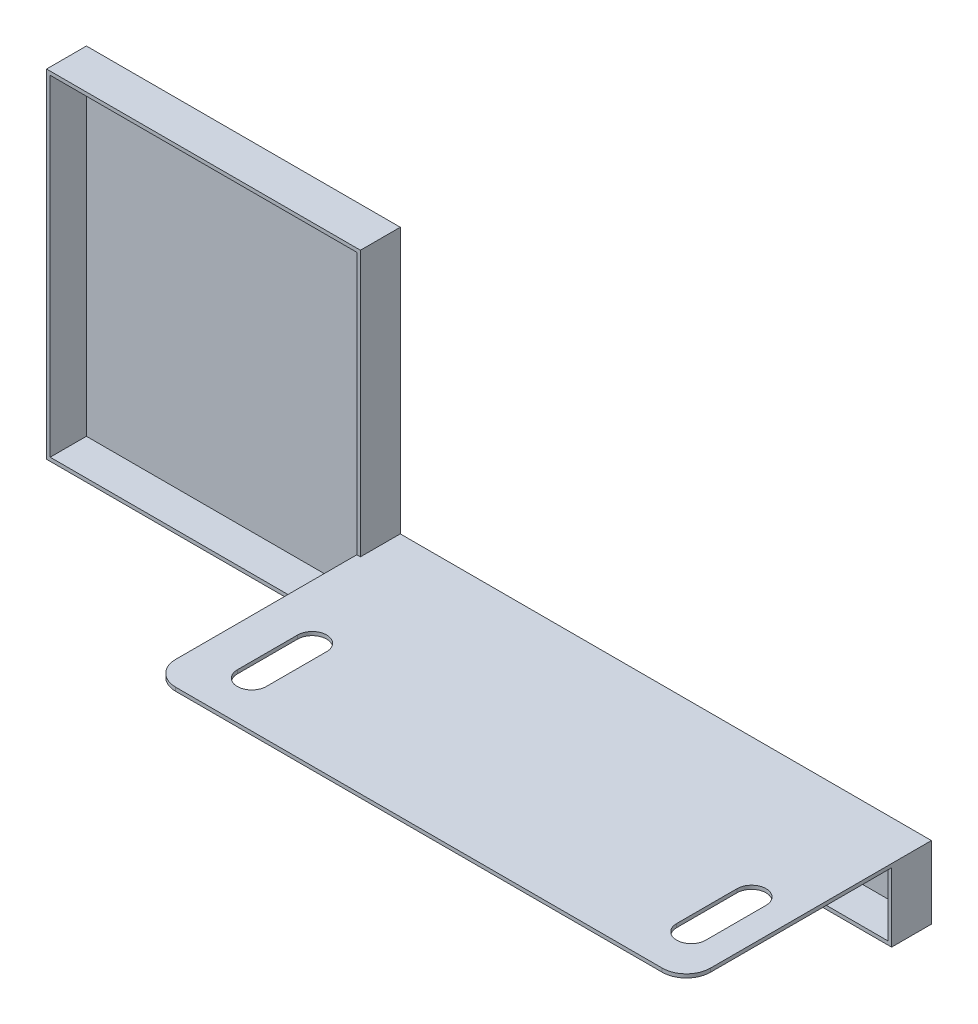
SolidWorks part; units mm, degrees
ref_plane "前视基准面" through (0, 0, 0) normal (0, 0, 1) x (1, 0, 0)
ref_plane "上视基准面" through (0, 0, 0) normal (0, 1, 0) x (1, 0, 0)
ref_plane "右视基准面" through (0, 0, 0) normal (1, 0, 0) x (0, 0, -1)
sketch "草图1" plane through (0, 0, 0) normal (0, 0, 1) x (1, 0, 0)
  line L1 (-175, 70) -> (175, 70)
  line L2 (-175, 70) -> (-175, -70)
  line L3 (-175, -70) -> (175, -70)
  line L4 (175, 70) -> (175, -70)
  line L5 (-175, 70) -> (175, -70) construction
  line L6 (-175, -70) -> (175, 70) construction
  point P0 (0, 0)
  dimension "D1" = 350
  dimension "D2" = 140
extrude "凸台-拉伸1" add sketch "草图1" along normal blind 1.5
sketch "草图2" plane through (0, 0, 1.5) normal (0, 0, 1) x (1, 0, 0)
  line L0 (-175, -70) -> (175, -70) construction
  line L1 (175, 70) -> (-45, 70)
  line L2 (175, 70) -> (175, -40)
  line L3 (175, -40) -> (-45, -40)
  line L4 (-45, 70) -> (-45, -40)
  dimension "D1" = 220
  dimension "D2" = 30
extrude "切除-拉伸1" cut sketch "草图2" against normal blind 2
sketch "草图3" plane through (0, 0, 1.5) normal (0, 0, 1) x (1, 0, 0)
  line L0 (-45, 70) -> (-45, -40) construction
  line L1 (175, -70) -> (175, -40) construction
  line L2 (-175, -70) -> (175, -70) construction
  line L3 (-175, 70) -> (-175, -70) construction
  line L4 (-45, 70) -> (-175, 70) construction
  line L5 (-45, 70) -> (-45, -40)
  line L6 (175, -70) -> (175, -40)
  line L7 (-175, -70) -> (175, -70)
  line L8 (-175, 70) -> (-175, -70)
  line L9 (-45, 70) -> (-175, 70)
extrude "拉伸-薄壁1" add sketch "草图3" along normal blind 15 thin
sketch "草图4" plane through (0, 0, 1.5) normal (0, 0, 1) x (1, 0, 0)
  line L1 (-46.5, -40) -> (175, -40)
  line L2 (-46.5, -40) -> (-46.5, -41.5)
  line L3 (-46.5, -41.5) -> (175, -41.5)
  line L4 (175, -40) -> (175, -41.5)
  line L5 (175, -70) -> (175, -40) construction
  dimension "D1" = 1.5
extrude "凸台-拉伸3" add sketch "草图4" along normal blind 100
fillet "圆角1" radius 10 2 edges at (175, -40.75, 101.5) (-46.5, -40.75, 101.5)
sketch "草图5" plane through (0, -41.5, 0) normal (0, -1, 0) x (1, 0, 0)
  line L0 (-24, 82.5) -> (-24, 57.5) construction
  line L1 (-18, 82.5) -> (-18, 57.5)
  line L2 (-30, 82.5) -> (-30, 57.5)
  line L3 (-24, 70) -> (158, 70) construction
  line L4 (158, 82.5) -> (158, 57.5) construction
  line L5 (164, 82.5) -> (164, 57.5)
  line L6 (152, 82.5) -> (152, 57.5)
  line L7 (175, 91.5) -> (175, 16.5) construction
  line L8 (-175, 0) -> (175, 0) construction
  arc A0 (-18, 82.5) -> (-30, 82.5) centre (-24, 82.5) ccw
  arc A1 (-30, 57.5) -> (-18, 57.5) centre (-24, 57.5) ccw
  arc A2 (164, 82.5) -> (152, 82.5) centre (158, 82.5) ccw
  arc A3 (152, 57.5) -> (164, 57.5) centre (158, 57.5) ccw
  point P2 (-24, 70)
  point P11 (158, 70)
  dimension "D1" = 12
  dimension "D2" = 25
  dimension "D3" = 182
  dimension "D4" = 17
  dimension "D5" = 70
extrude "切除-拉伸2" cut sketch "草图5" against normal blind 100
